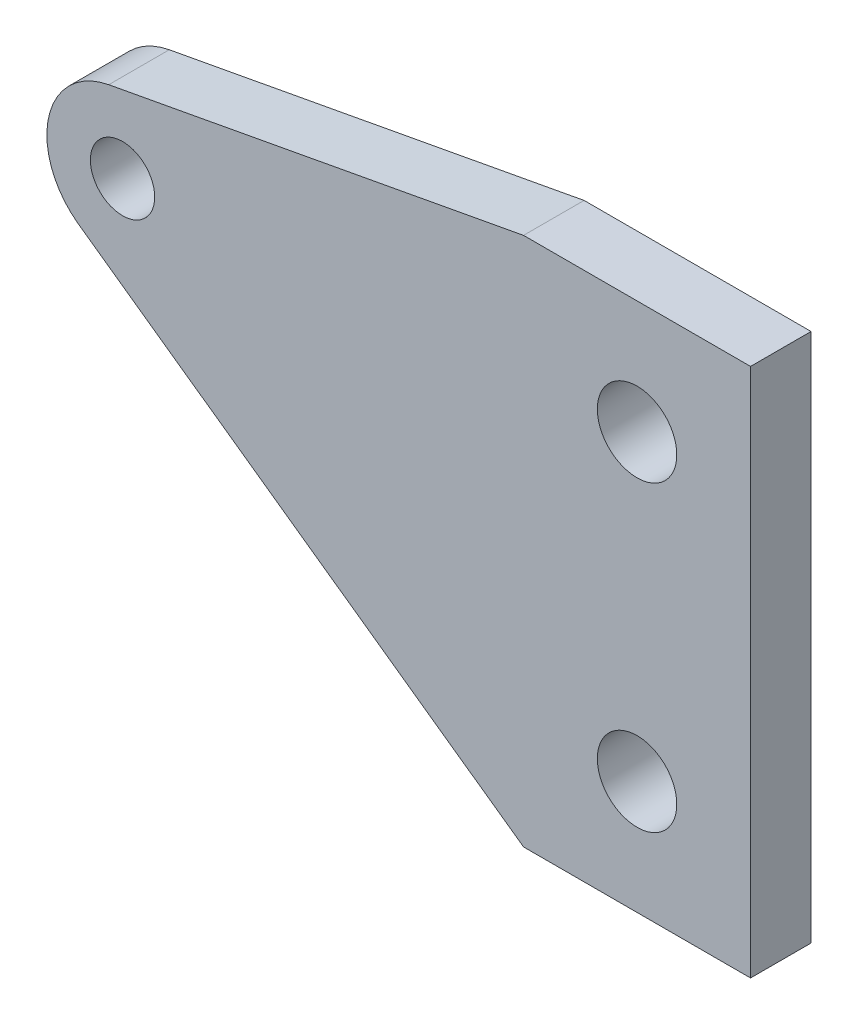
SolidWorks part; units mm, degrees
material "1023 碳钢板 (SS)"
ref_plane "Front Plane" through (0, 0, 0) normal (0, 0, 1) x (1, 0, 0)
ref_plane "Top Plane" through (0, 0, 0) normal (0, 1, 0) x (1, 0, 0)
ref_plane "Right Plane" through (0, 0, 0) normal (1, 0, 0) x (0, 0, -1)
ref_plane "Plane4" through (0, 0, 4) normal (0, 0, 1) x (1, 0, 0)
sketch "Sketch1" plane through (0, 0, 4) normal (0, 0, 1) x (1, 0, 0)
  line L0 (55.6136, -36.5909) -> (55.6136, 33.4091)
  line L1 (55.6136, 33.4091) -> (-44.3864, 33.4091)
  line L2 (-44.3864, 33.4091) -> (-44.3864, -36.5909)
  line L3 (-44.3864, -36.5909) -> (55.6136, -36.5909)
  circle A0 centre (40.6136, -21.5909) radius 5.25
  circle A1 centre (40.6136, 18.4091) radius 5.25
  dimension "D1" = 10.5
  dimension "D2" = 10.5
  dimension "D4" = 15
  dimension "D6" = 15
  dimension "D7" = 15
  dimension "D3" = 100
  dimension "D5" = 70
extrude "Boss-Extrude1" add sketch "Sketch1" against normal blind 8
sketch "Sketch2" plane through (0, 0, 4) normal (0, 0, 1) x (1, 0, 0)
  line L2 (55.6136, 33.4091) -> (-44.3864, 33.4091) construction
  line L3 (-44.3864, -36.5909) -> (55.6136, -36.5909) construction
  line L4 (25.6136, 33.4091) -> (-29.2099, 23.2414)
  line L5 (-33.1853, 5.2622) -> (25.6136, -36.5909)
  line L6 (25.6136, -36.5909) -> (55.6136, -36.5909)
  line L7 (55.6136, -36.5909) -> (55.6136, 33.4091)
  line L8 (55.6136, 33.4091) -> (25.6136, 33.4091)
  circle A1 centre (40.6136, 18.4091) radius 5.25 construction
  arc A2 (-29.2099, 23.2414) -> (-33.1853, 5.2622) centre (-27.3864, 13.4091) ccw
  dimension "D1" = 30
  dimension "D2" = 30
  dimension "D3" = 83
  dimension "D4" = 20
  dimension "D5" = 5
extrude "Cut-Extrude1" cut sketch "Sketch2" against normal blind 10 flip side to cut
sketch "Sketch3" plane through (0, 0, 4) normal (0, 0, 1) x (1, 0, 0)
  line L0 (55.6136, -36.5909) -> (55.6136, 33.4091) construction
  circle A0 centre (-27.3864, 13.4091) radius 6.1763
  circle A1 centre (40.6136, 18.4091) radius 5.25 construction
  dimension "D1" = 5
  dimension "D2" = 83
hole_wizard "M10 Tapped Hole1" positions "Sketch4" profile "Sketch5" tap size "M10" standard "GB"
sketch "Sketch4" plane through (0, 0, 4) normal (0, 0, 1) x (1, 0, 0)
  point P0 (-27.3864, 13.4091)
sketch "Sketch5" plane through (-27.3864, 13.4091, 4) normal (1, 0, 0) x (0, -1, 0)
  line L0 (0, 0) -> (0, 27.0537)
  line L1 (0, 27.0537) -> (4.25, 24.5)
  line L2 (4.25, 24.5) -> (4.25, 0)
  line L5 (4.25, 0) -> (0, 0)
  line L10 (0, 27.0537) -> (-4.25, 24.5) construction
  line L11 (0, -6.35) -> (0, 107.95) construction
  dimension "螺纹孔钻头直径" = 8.5
  dimension "螺纹孔钻头深度" = 24.5
  dimension "导头角度" = 118
cosmetic thread "Cosmetic Thread1"
